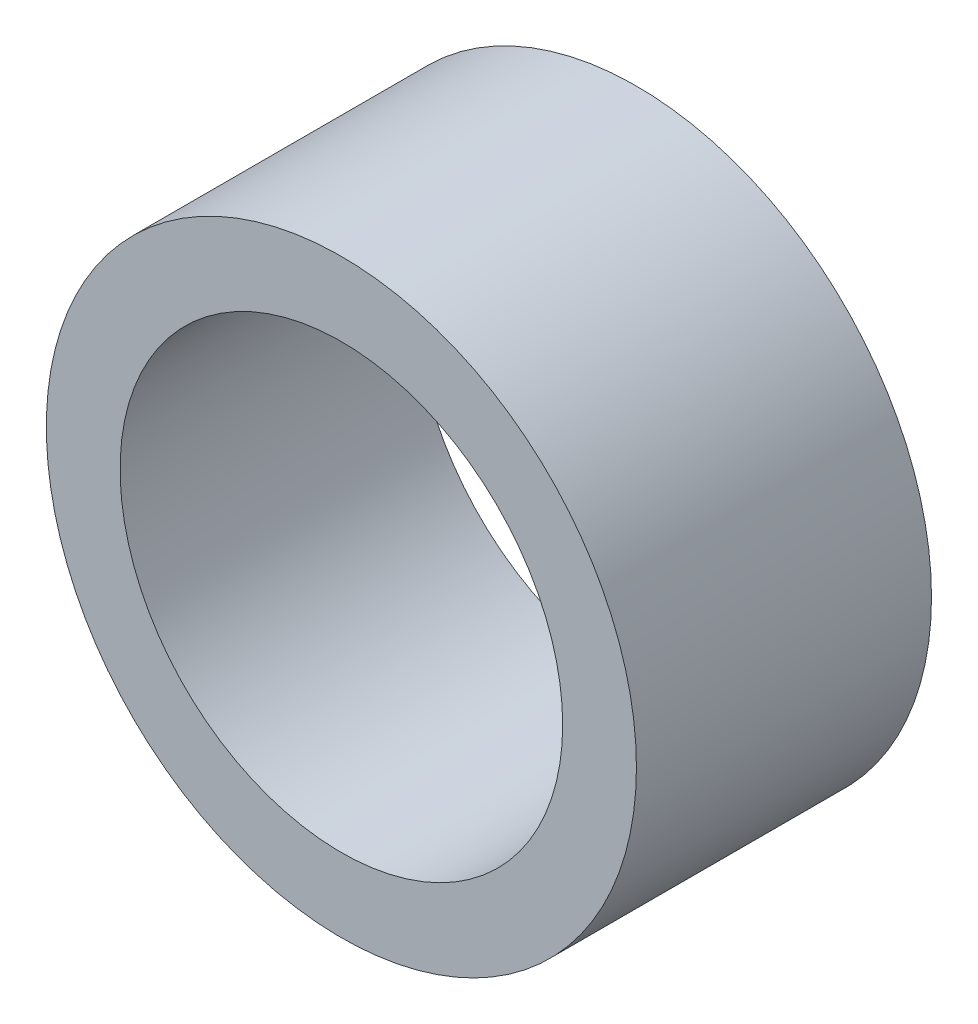
SolidWorks part; units mm, degrees
ref_plane "Front Plane" through (0, 0, 0) normal (0, 0, 1) x (1, 0, 0)
ref_plane "Top Plane" through (0, 0, 0) normal (0, 1, 0) x (1, 0, 0)
ref_plane "Right Plane" through (0, 0, 0) normal (1, 0, 0) x (0, 0, -1)
sketch "Sketch2" plane through (0, 0, 0) normal (0, 0, 1) x (1, 0, 0)
  circle A0 centre (0, 0) radius 4
  circle A1 centre (0, 0) radius 3
  dimension "D1" = 6
  dimension "D2" = 8
extrude "Boss-Extrude1" add sketch "Sketch2" along normal blind 4
